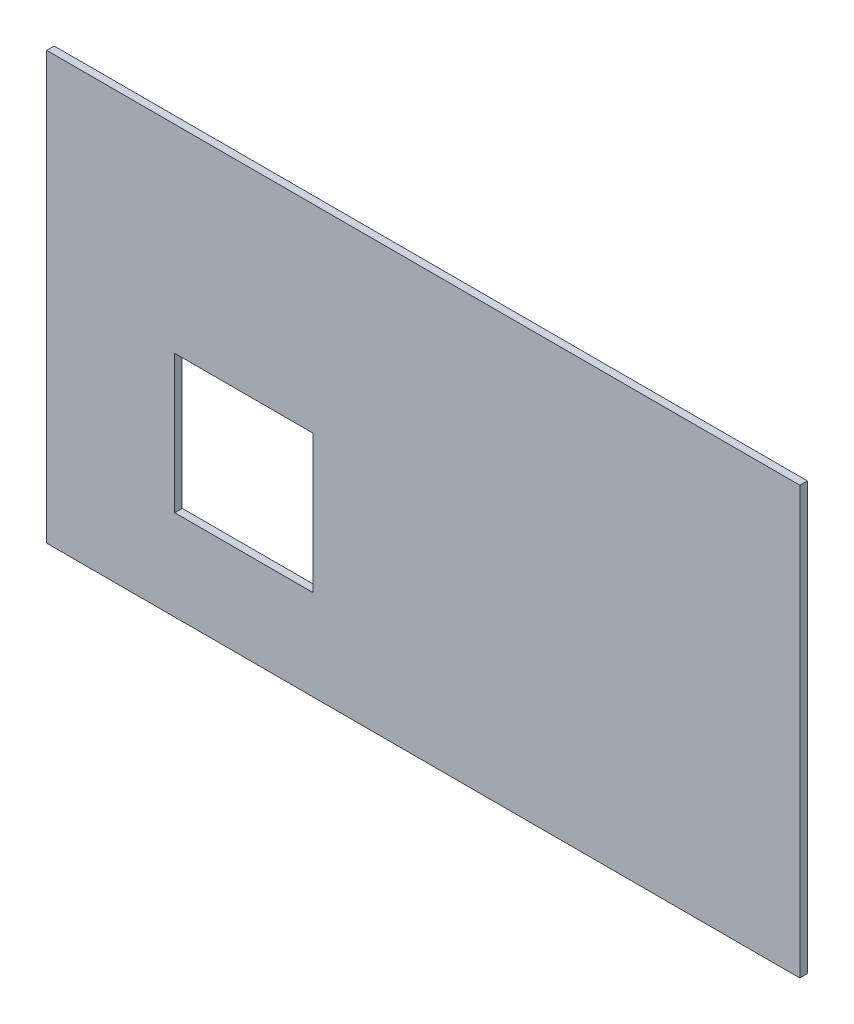
SolidWorks part; units mm, degrees
ref_plane "Front Plane" through (0, 0, 0) normal (0, 0, 1) x (1, 0, 0)
ref_plane "Top Plane" through (0, 0, 0) normal (0, 1, 0) x (1, 0, 0)
ref_plane "Right Plane" through (0, 0, 0) normal (1, 0, 0) x (0, 0, -1)
sketch "Sketch1" plane through (0, 0, 0) normal (0, 0, 1) x (1, 0, 0)
  line L0 (0, 0) -> (-20, 0) construction
  line L2 (-170, 85) -> (130, 85)
  line L3 (-170, 85) -> (-170, -85)
  line L4 (-170, -85) -> (130, -85)
  line L5 (130, 85) -> (130, -85)
  line L6 (-170, 85) -> (130, -85) construction
  line L7 (-170, -85) -> (130, 85) construction
  dimension "D1" = 300
  dimension "D2" = 170
  dimension "D3" = 20
extrude "Boss-Extrude1" add sketch "Sketch1" along normal blind 3
sketch "Sketch2" plane through (0, 0, 0) normal (0, 0, -1) x (-1, 0, 0)
  line L1 (119, -49) -> (119, 6)
  line L3 (64, -49) -> (119, -49)
  line L5 (64, 6) -> (64, -49)
  line L7 (119, 6) -> (64, 6)
extrude "Cut-Extrude2" cut sketch "Sketch2" against normal blind 40.5
